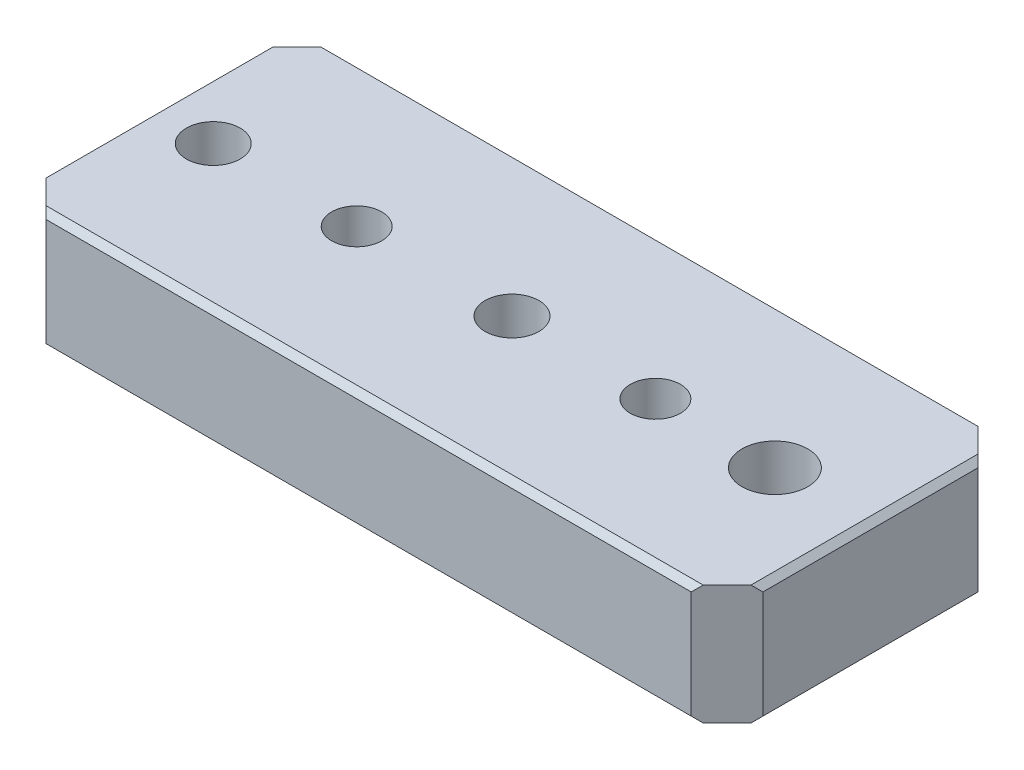
from build123d import *

# Parameters (mm, degrees)
SKETCH1_W                                          = 55
SKETCH1_H                                          = 24
BOSS_EXTRUDE1_DEPTH                                = 10
HOLE_WIZARD_3_D                                    = 4.5
HOLE_WIZARD_3_DEPTH                                = 12.4
HOLE_WIZARD_3_CBORE_D                              = 8
HOLE_WIZARD_3_CBORE_DEPTH                          = 4.6
HOLE_WIZARD_3_TIP                                  = 1.351936393
SKETCH6_W                                          = 5
SKETCH6_H                                          = 24
BOSS_EXTRUDE2_DEPTH                                = 10
CHAMFER1_SIZE                                      = 3
CHAMFER2_SIZE                                      = 0.5
HOLE_SIZE_BASED_ON_SOCKET_HEAD_CAP_SCR_D           = 5.5
HOLE_SIZE_BASED_ON_SOCKET_HEAD_CAP_SCR_DEPTH       = 12.4
HOLE_SIZE_BASED_ON_SOCKET_HEAD_CAP_SCR_CBORE_D     = 10
HOLE_SIZE_BASED_ON_SOCKET_HEAD_CAP_SCR_CBORE_DEPTH = 5.7
HOLE_SIZE_BASED_ON_SOCKET_HEAD_CAP_SCR_TIP         = 1.652366702
M5_TAPPED_HOLE1_D                                  = 4.2


with BuildPart() as part:
    # Sketch1 → Boss-Extrude1 (new body)
    with BuildSketch(Plane(origin=(0, 0, 0), x_dir=(1, 0, 0), z_dir=(0, 1, 0))):
        with Locations((-1.42708605, -3.163732927)):
            Rectangle(SKETCH1_W, SKETCH1_H)
    extrude(amount=BOSS_EXTRUDE1_DEPTH)

    # 打孔尺寸(%根据)内六角圆柱头螺钉的类型3
    with Locations(Plane(origin=(0, 0, 0), x_dir=(-1, 0, 0), z_dir=(0, -1, 0))):
        with Locations((23.92708605, -3.163732927), (-1.07291395, -3.163732927)):
            CounterBoreHole(HOLE_WIZARD_3_D / 2, HOLE_WIZARD_3_CBORE_D / 2, HOLE_WIZARD_3_CBORE_DEPTH, depth=HOLE_WIZARD_3_DEPTH)
            with Locations((0, 0, -(HOLE_WIZARD_3_DEPTH + HOLE_WIZARD_3_TIP / 2))):  # 118° drill point
                Cone(0, HOLE_WIZARD_3_D / 2, HOLE_WIZARD_3_TIP, mode=Mode.SUBTRACT)

    # Sketch6 → Boss-Extrude2 (add)
    with BuildSketch(Plane.XZ):
        with Locations((28.57291395, 3.163732927)):
            Rectangle(SKETCH6_W, SKETCH6_H)
    extrude(amount=-BOSS_EXTRUDE2_DEPTH)

    # Chamfer1
    chamfer1_edges = [part.edges().sort_by_distance(p)[0] for p in [
        (31.07291395, 5, 15.163732927),
        (31.07291395, 5, -8.836267073),
        (-28.92708605, 5, -8.836267073),
        (-28.92708605, 5, 15.163732927),
    ]]
    chamfer(chamfer1_edges, length=CHAMFER1_SIZE)

    # Chamfer2
    chamfer2_edges = [part.edges().sort_by_distance(p)[0] for p in [
        (1.07291395, 0, -8.836267073),
        (1.07291395, 10, -8.836267073),
        (-28.92708605, 0, 3.163732927),
        (31.07291395, 0, 3.163732927),
        (1.07291395, 0, 15.163732927),
        (31.07291395, 10, 3.163732927),
        (-28.92708605, 10, 3.163732927),
        (1.07291395, 10, 15.163732927),
    ]]
    chamfer(chamfer2_edges, length=CHAMFER2_SIZE)

    # Hole Size _Based On_ Socket Head Cap Scr
    with Locations(Plane(origin=(0, 0, 0), x_dir=(-1, 0, 0), z_dir=(0, -1, 0))):
        with Locations((-23.07291395, -3.163732927)):
            CounterBoreHole(HOLE_SIZE_BASED_ON_SOCKET_HEAD_CAP_SCR_D / 2, HOLE_SIZE_BASED_ON_SOCKET_HEAD_CAP_SCR_CBORE_D / 2, HOLE_SIZE_BASED_ON_SOCKET_HEAD_CAP_SCR_CBORE_DEPTH, depth=HOLE_SIZE_BASED_ON_SOCKET_HEAD_CAP_SCR_DEPTH)
            with Locations((0, 0, -(HOLE_SIZE_BASED_ON_SOCKET_HEAD_CAP_SCR_DEPTH + HOLE_SIZE_BASED_ON_SOCKET_HEAD_CAP_SCR_TIP / 2))):  # 118° drill point
                Cone(0, HOLE_SIZE_BASED_ON_SOCKET_HEAD_CAP_SCR_D / 2, HOLE_SIZE_BASED_ON_SOCKET_HEAD_CAP_SCR_TIP, mode=Mode.SUBTRACT)

    # M5 Tapped Hole1 (through all)
    with Locations(Plane(origin=(0, 10, 0), x_dir=(1, 0, 0), z_dir=(0, 1, 0))):
        with Locations((-11.92708605, -3.163732927), (13.07291395, -3.163732927)):
            Hole(M5_TAPPED_HOLE1_D / 2)


solid = part.part
